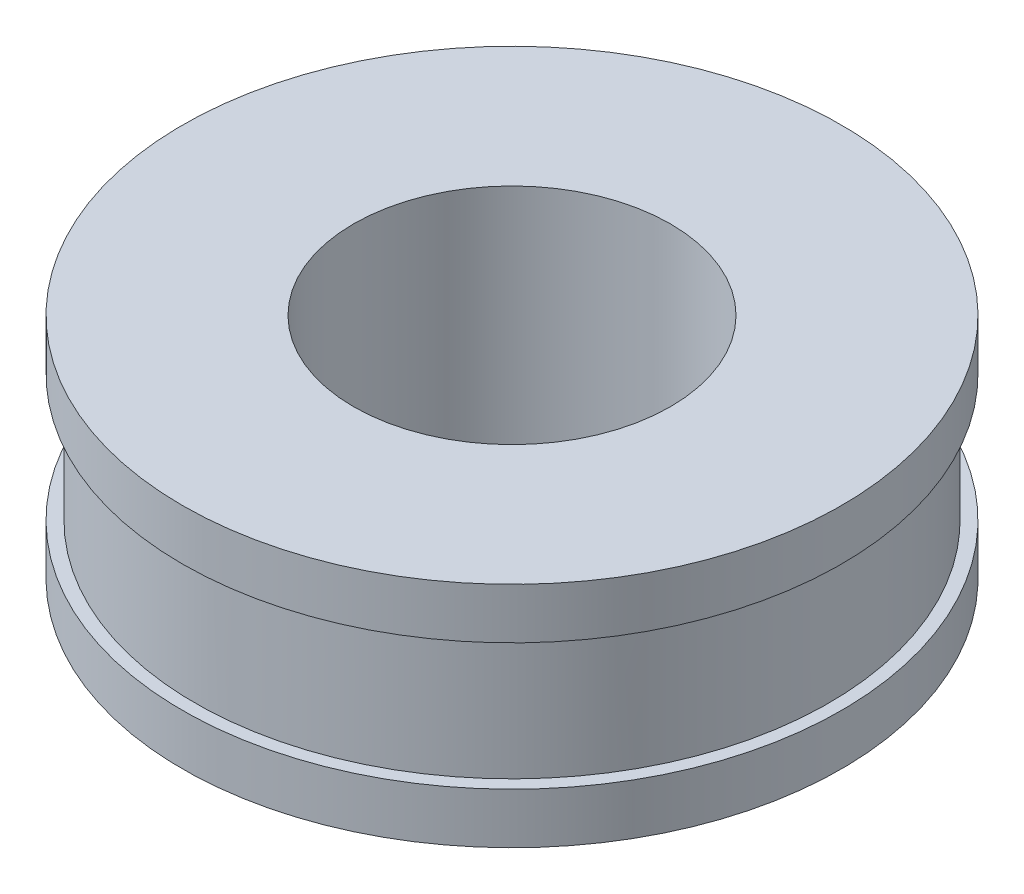
from build123d import *

# Parameters (mm, degrees)
SKETCH1_R           = 50
BOSS_EXTRUDE1_DEPTH = 20
SKETCH2_R           = 52
BOSS_EXTRUDE2_DEPTH = 8
BOSS_EXTRUDE3_START = 8
SKETCH3_R           = 52
BOSS_EXTRUDE3_DEPTH = 8
SKETCH4_R           = 25
CUT_EXTRUDE1_DEPTH  = 82.877957962


with BuildPart() as part:
    # Sketch1 → Boss-Extrude1 (new body)
    with BuildSketch(Plane(origin=(0, 0, 0), x_dir=(1, 0, 0), z_dir=(0, 1, 0))):
        with Locations(Location((0, 0, 0), (0, 0, 270))):
            Circle(SKETCH1_R)
    extrude(amount=BOSS_EXTRUDE1_DEPTH)

    # Sketch2 → Boss-Extrude2 (add)
    with BuildSketch(Plane(origin=(0, 20, 0), x_dir=(1, 0, 0), z_dir=(0, 1, 0))):
        with Locations(Location((0, 0, 0), (0, 0, 270))):
            Circle(SKETCH2_R)
    extrude(amount=BOSS_EXTRUDE2_DEPTH)

    # Sketch3 → Boss-Extrude3 (add)
    with BuildSketch(Plane.XZ.offset(BOSS_EXTRUDE3_START)):
        with Locations(Location((0, 0, 0), (0, 0, 90))):
            Circle(SKETCH3_R)
    extrude(amount=-BOSS_EXTRUDE3_DEPTH)

    # Sketch4 → Cut-Extrude1 (cut, through all)
    with BuildSketch(Plane.XZ.offset(8)):
        with Locations(Location((0, 0, 0), (0, 0, 270))):
            Circle(SKETCH4_R)
    extrude(amount=-CUT_EXTRUDE1_DEPTH, mode=Mode.SUBTRACT)


solid = part.part
